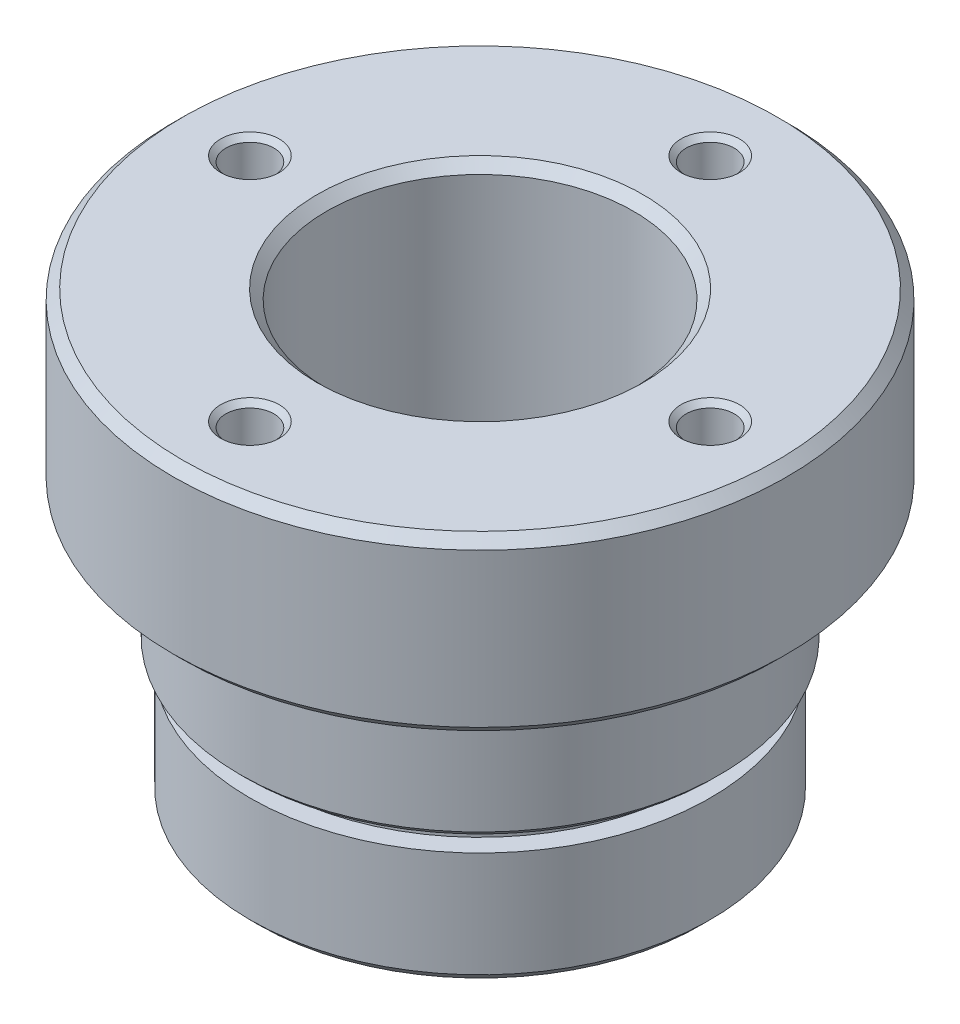
SolidWorks part; units mm, degrees
material "SUS 303"
ref_plane "Front Plane" through (0, 0, 0) normal (0, 0, 1) x (1, 0, 0)
ref_plane "Top Plane" through (0, 0, 0) normal (0, 1, 0) x (1, 0, 0)
ref_plane "Right Plane" through (0, 0, 0) normal (1, 0, 0) x (0, 0, -1)
sketch "Sketch1" plane through (0, 0, 0) normal (0, 0, 1) x (1, 0, 0)
  line L0 (8.5, 0) -> (15.5, 0)
  line L1 (16, -0.5) -> (16, -8.5)
  line L2 (15.5, -9) -> (12, -9)
  line L3 (12.5, -9.7) -> (12.5, -15.7)
  line L9 (8, -22.5) -> (8, -0.5)
  line L10 (0, 0) -> (0, -26.5698) construction
  line L13 (8, -0.5) -> (8.5, 0)
  line L14 (15.5, 0) -> (16, -0.5)
  line L15 (16, -8.5) -> (15.5, -9)
  line L20 (12.2, -16) -> (11, -16)
  line L23 (12, -17) -> (12, -22.5)
  line L25 (12.5, -15.7) -> (12.2, -16)
  line L26 (12.5, -9.7) -> (12, -9.2)
  line L27 (12, -9.2) -> (12, -9)
  line L32 (8.5, -23) -> (11.5, -23)
  line L34 (11, -16) -> (11, -17)
  line L35 (11, -17) -> (12, -17)
  line L36 (8, -22.5) -> (8.5, -23)
  line L37 (11.5, -23) -> (12, -22.5)
  point P0 (8, 0)
  point P1 (16, 0)
  point P3 (8, -23)
  point P4 (16, -9)
  point P7 (12.5, -16)
  point P8 (12, -23)
  dimension "D1" = 16
  dimension "D2" = 25
  dimension "D3" = 32
  dimension "D4" = 7
  dimension "D5" = 16
  dimension "D6" = 23
  dimension "D7" = 24
  dimension "D8" = 1
  dimension "D10" = 1
  dimension "D17" = 0.5
  dimension "D21" = 135
  dimension "D23" = 0.2
revolve "Revolve1" add sketch "Sketch1" angle 360 about L10
cosmetic thread "Cosmetic Thread1"
hole_wizard "M3 Tapped Hole1" positions "Sketch2" profile "Sketch3" tap size "M3" standard "GB"
sketch "Sketch2" plane through (0, 0, 0) normal (0, 1, 0) x (1, 0, 0)
  line L0 (-12, 0) -> (0, 0)
  line L1 (0, 12) -> (0, 0)
  line L3 (12, 0) -> (0, 0)
  line L5 (0, -12) -> (0, 0)
  point P0 (-12, 0)
  point P8 (0, 12)
  point P10 (12, 0)
  point P12 (0, -12)
  dimension "D1" = 12
sketch "Sketch3" plane through (-12, 0, 0) normal (1, 0, 0) x (0, 0, 1)
  line L0 (0, 0) -> (0, 7.7511)
  line L1 (0, 7.7511) -> (1.25, 7)
  line L2 (1.25, 7) -> (1.25, 0.275)
  line L3 (1.25, 0.275) -> (1.525, 0)
  line L5 (1.525, 0) -> (0, 0)
  line L6 (-1.25, 0.275) -> (-1.525, 0) construction
  line L10 (0, 7.7511) -> (-1.25, 7) construction
  line L11 (0, -6.35) -> (0, 107.95) construction
  dimension "螺纹孔钻头直径" = 2.5
  dimension "螺纹孔钻头深度" = 7
  dimension "近端锥形沉头孔直径" = 3.05
  dimension "近端锥形沉头孔角度" = 90
  dimension "导头角度" = 118
cosmetic thread "孔螺蚊线1"
cosmetic thread "Cosmetic Thread2"
cosmetic thread "Cosmetic Thread3"
cosmetic thread "Cosmetic Thread4"
